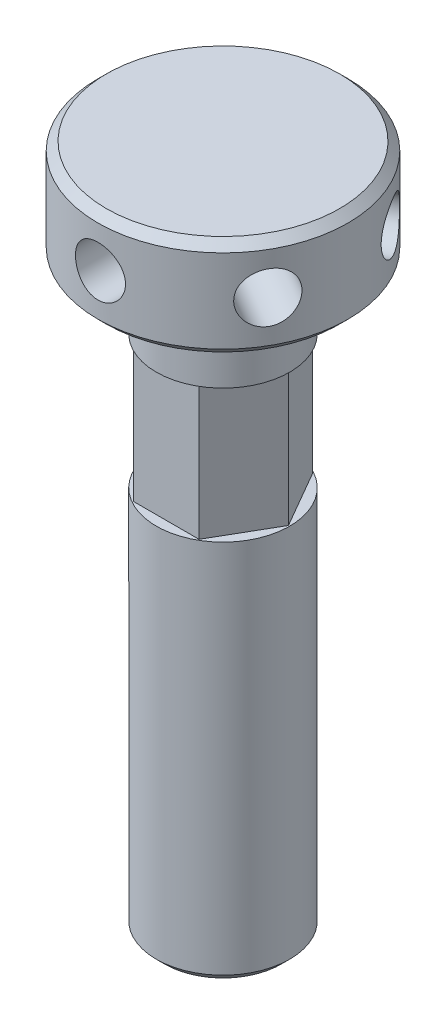
SolidWorks part; units mm, degrees
ref_plane "Front Plane" through (0, 0, 0) normal (0, 0, 1) x (1, 0, 0)
ref_plane "Top Plane" through (0, 0, 0) normal (0, 1, 0) x (1, 0, 0)
ref_plane "Right Plane" through (0, 0, 0) normal (1, 0, 0) x (0, 0, -1)
sketch "Sketch1" plane through (0, 0, 0) normal (0, 1, 0) x (1, 0, 0)
  circle A0 centre (0, 0) radius 4
  dimension "D1" = 8
extrude "Boss-Extrude1" add sketch "Sketch1" along normal blind 35
cosmetic thread "Cosmetic Thread1" parameters "D1"=20, "D2"=7.5
sketch "Sketch2" plane through (0, 35, 0) normal (0, 1, 0) x (1, 0, 0)
  circle A0 centre (0, 0) radius 7.5
  dimension "D1" = 15
extrude "Boss-Extrude2" add sketch "Sketch2" along normal blind 6
chamfer "Chamfer1" distance 0.5 angle 45 3 edges at (0, 0, 4) (0, 35, 7.5) (0, 41, 7.5)
sketch "Sketch3" plane through (0, 0, 0) normal (0, 0, 1) x (1, 0, 0)
  line L0 (-7.5, 38) -> (49992.5, 38) construction
  line L1 (-7.5, 40.5) -> (-7.5, 35.5) construction
  line L2 (0, 41) -> (0, -49959) construction
  line L3 (7, 41) -> (-7, 41) construction
  circle A0 centre (0, 38) radius 1.5
  point P4 (-7.5, 38)
  point P9 (0, 41)
  dimension "D1" = 3
extrude "Cut-Extrude1" cut sketch "Sketch3" against normal mid plane 19
pattern_circular "CirPattern1" count 6 over 360 about axis through (0, 41, 0) along (0, -1, 0) of "Cut-Extrude1"
sketch "Sketch5" plane through (0, 0, 0) normal (1, 0, 0) x (0, 0, -1)
  line L0 (4, 0.5) -> (4, 35) construction
  line L1 (3.4, 31) -> (4.6, 31)
  line L2 (3.4, 31) -> (3.4, 23)
  line L3 (3.4, 23) -> (4.6, 23)
  line L4 (4.6, 31) -> (4.6, 23)
  line L5 (3.4, 31) -> (4.6, 23) construction
  line L6 (3.4, 23) -> (4.6, 31) construction
  line L7 (7, 41) -> (-7, 41) construction
  point P0 (4, 27)
  dimension "D1" = 8
  dimension "D2" = 10
  dimension "D3" = 0.6
extrude "Cut-Extrude3" cut sketch "Sketch5" against normal mid plane 10
pattern_circular "CirPattern3" count 6 over 360 about axis through (0, 0, 0) along (0, 1, 0) of "Cut-Extrude3"
